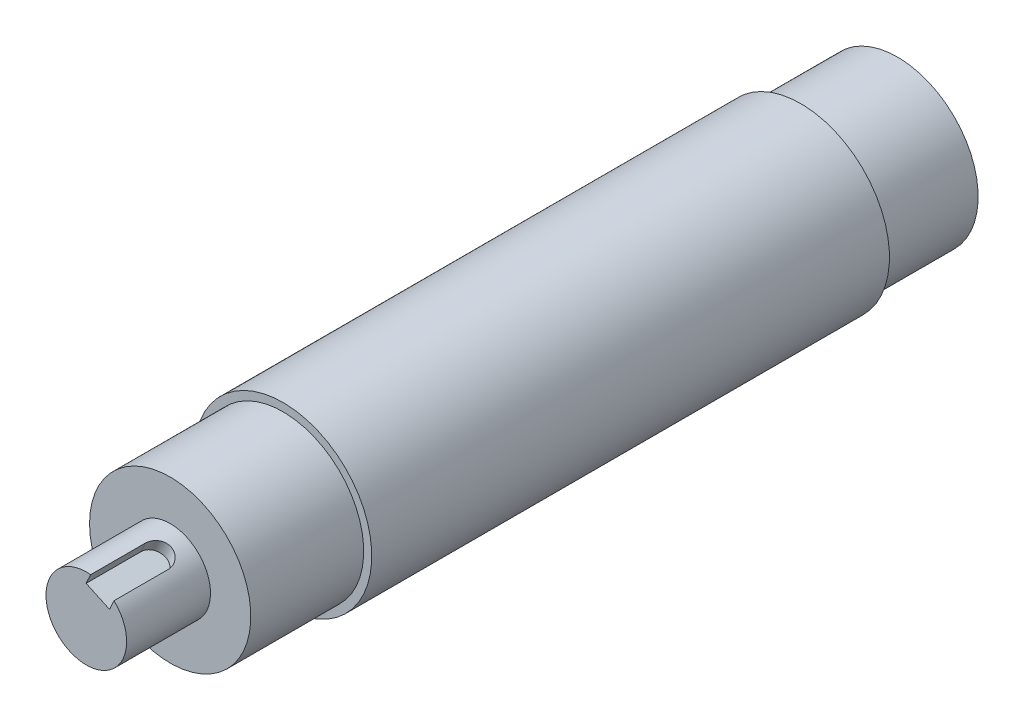
SolidWorks part; units mm, degrees
ref_plane "前视基准面" through (0, 0, 0) normal (0, 0, 1) x (1, 0, 0)
ref_plane "上视基准面" through (0, 0, 0) normal (0, 1, 0) x (1, 0, 0)
ref_plane "右视基准面" through (0, 0, 0) normal (1, 0, 0) x (0, 0, -1)
sketch "草图1" plane through (0, 0, 0) normal (0, 1, 0) x (1, 0, 0)
  line L0 (0, 0) -> (0, -80836.6018) construction
  line L4 (-25, 34) -> (-25, 4)
  line L5 (-25, 4) -> (-27.5, 4)
  line L6 (-27.5, 4) -> (-27.5, -156.5)
  line L7 (-27.5, -156.5) -> (-25, -156.5)
  line L8 (-25, -156.5) -> (-25, -191.5)
  line L9 (-25, -191.5) -> (-12.5, -191.5)
  line L10 (-12.5, -191.5) -> (-12.5, -217.5)
  line L11 (-12.5, -217.5) -> (0, -217.5)
  line L12 (0, -217.5) -> (0, 34)
  line L13 (-25, 34) -> (0, 34)
  point P4 (0, 77.933)
  dimension "D1" = 12.5
  dimension "D3" = 30
  dimension "D4" = 55
  dimension "D5" = 50
  dimension "D6" = 217.5
  dimension "D7" = 35
  dimension "D8" = 26
  dimension "D9" = 160.5
revolve "旋转1" add sketch "草图1" angle 360 about L0
ref_plane "基准面2" through (0, -27.5, 0) normal (0, -1, 0) x (-1, 0, 0)
sketch "草图3" plane through (0, -27.5, 0) normal (0, -1, 0) x (-1, 0, 0)
  line L0 (0, -66.5) -> (0, -112.5) construction
  line L1 (8, -66.5) -> (8, -112.5)
  line L2 (-8, -66.5) -> (-8, -112.5)
  line L3 (-12.5, -217.5) -> (12.5, -217.5) construction
  line L4 (25, 34) -> (-25, 34) construction
  arc A0 (8, -66.5) -> (-8, -66.5) centre (0, -66.5) ccw
  arc A1 (-8, -112.5) -> (8, -112.5) centre (0, -112.5) ccw
  point P2 (0, -89.5)
  dimension "D2" = 105
  dimension "D3" = 92.5
  dimension "D1" = 16
extrude "切除-拉伸2" cut sketch "草图3" against normal blind 6
sketch "草图4" plane through (6.6271, 14.343, 0) normal (-0.4194, -0.9078, 0) x (0.9078, -0.4194, 0)
  line L0 (0, 219.3535) -> (0, 200.5) construction
  line L1 (4, 219.3535) -> (4, 200.5)
  line L2 (-4, 219.3535) -> (-4, 200.5)
  line L3 (12.5, 191.5) -> (-12.5, 191.5) construction
  arc A0 (4, 219.3535) -> (-4, 219.3535) centre (0, 219.3535) ccw
  arc A1 (-4, 200.5) -> (4, 200.5) centre (0, 200.5) ccw
  point P2 (0, 209.9267)
  dimension "D2" = 5
  dimension "D1" = 8
extrude "切除-拉伸3" cut sketch "草图4" along normal blind 7.3
